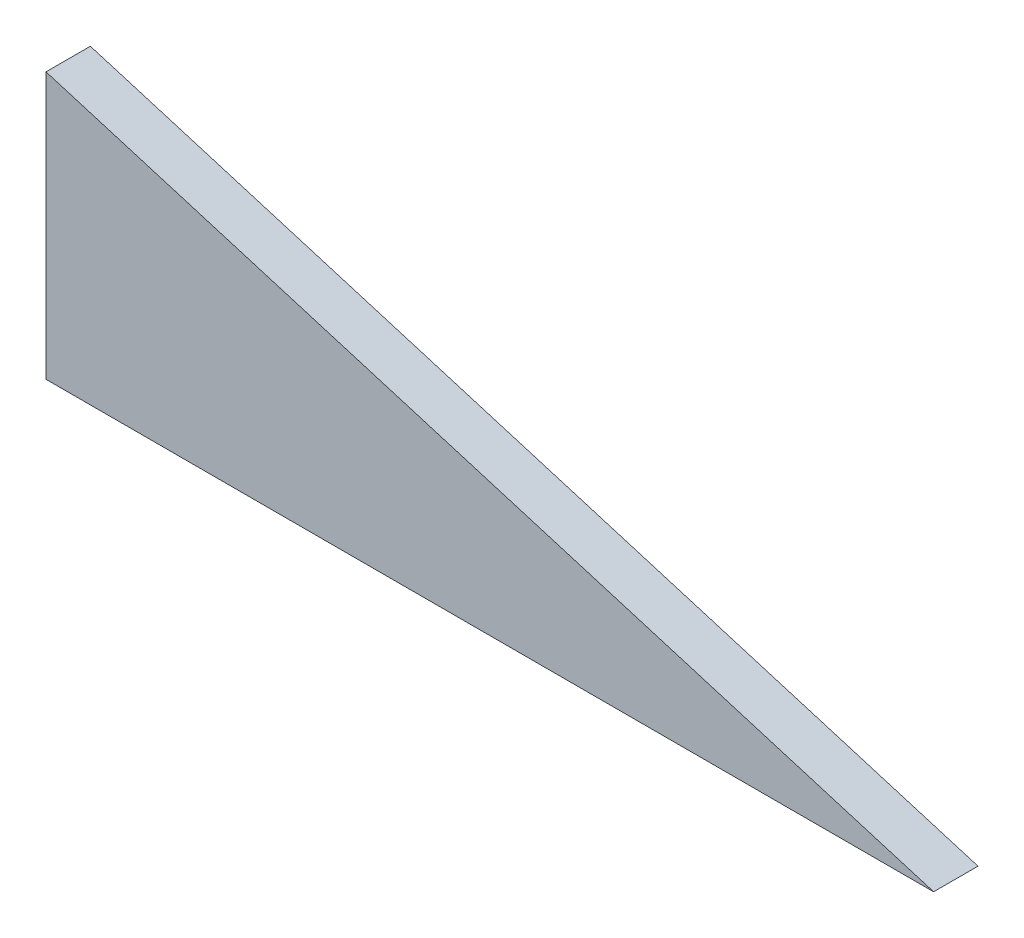
from build123d import *

# Parameters (mm, degrees)
EXTRUDE_1_DEPTH = 5


with BuildPart() as part:
    # 草图1 → 凸台-拉伸1 (new body)
    with BuildSketch(Plane.XY):
        Polygon((0, 0), (0, 30), (100, 0), align=None)
    extrude(amount=EXTRUDE_1_DEPTH)


solid = part.part
